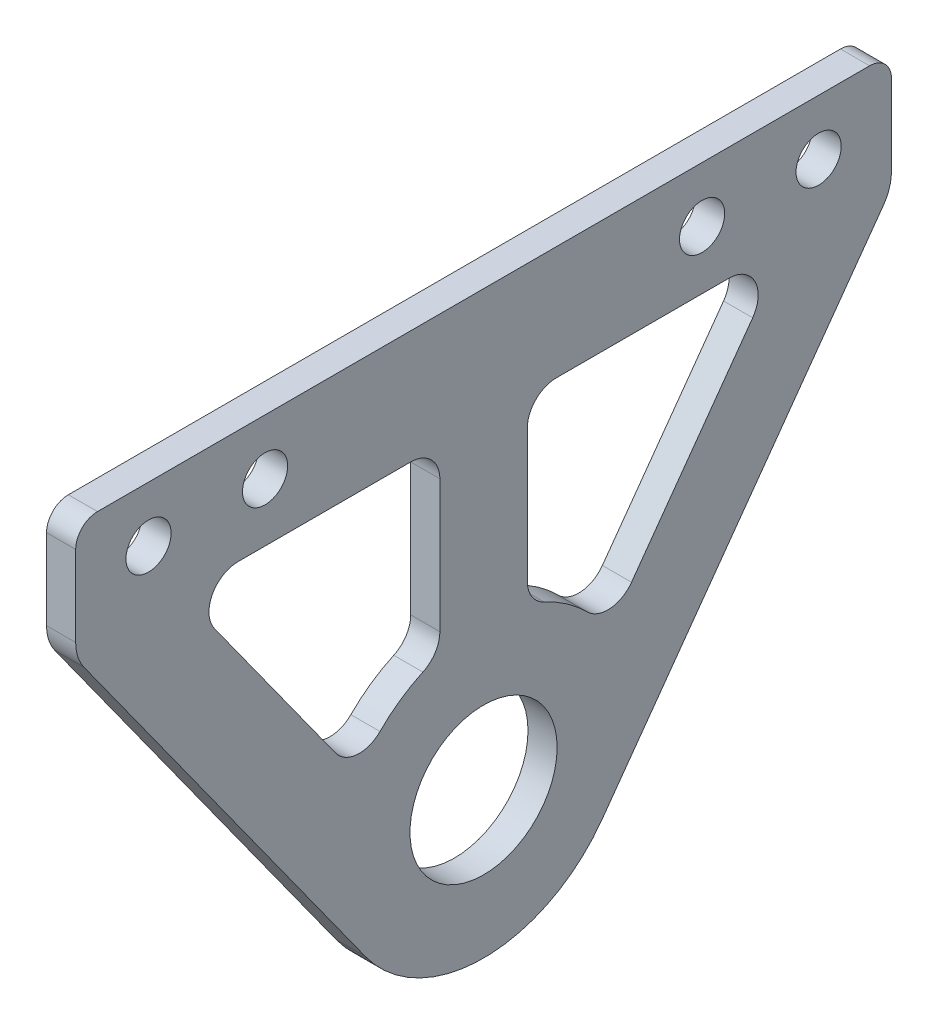
from build123d import *

# Parameters (mm, degrees)
SKETCH_1_R          = 5.05
SKETCH_1_R_2        = 1.55
EXTRUDE_1_DEPTH     = 2
CUT_EXTRUDE_1_DEPTH = 41.93946751
FILLET_1_R          = 2
FILLET_2_R          = 2
FILLET_3_R          = 3
FILLET_4_R          = 1.5


with BuildPart() as part:
    # 草图1 → 凸台-拉伸1 (new body)
    with BuildSketch(Plane(origin=(0, 0, 0), x_dir=(0, 0, -1), z_dir=(1, 0, 0))):
        with BuildLine():
            Line((-28, 29.8), (-28, 21.8))
            Line((-28, 21.8), (-8.117896343, -5.83949989))
            ThreePointArc((-8.117896343, -5.83949989), (0, -10), (8.117896343, -5.83949989))
            Line((8.117896343, -5.83949989), (28, 21.8))
            Line((28, 21.8), (28, 29.8))
            Line((28, 29.8), (-28, 29.8))
        make_face()
        Circle(SKETCH_1_R, mode=Mode.SUBTRACT)
        with Locations((-15, 26)):
            Circle(SKETCH_1_R_2, mode=Mode.SUBTRACT)
        with Locations((-23, 26)):
            Circle(SKETCH_1_R_2, mode=Mode.SUBTRACT)
        with Locations(Location((23, 26, 0), (0, 0, 180))):
            Circle(SKETCH_1_R_2, mode=Mode.SUBTRACT)
        with Locations(Location((15, 26, 0), (0, 0, 180))):
            Circle(SKETCH_1_R_2, mode=Mode.SUBTRACT)
    extrude(amount=EXTRUDE_1_DEPTH)

    # 草图2 → 切除-拉伸1 (cut, through all)
    with BuildSketch(Plane(origin=(0, 0, 0), x_dir=(0, 0, -1), z_dir=(1, 0, 0))):
        with BuildLine():
            Line((-3, 22), (-3, 9.539392014))
            ThreePointArc((-3, 9.539392014), (-6.209058392, 7.838851566), (-8.599148591, 5.104374939))
            Line((-8.599148591, 5.104374939), (-20.752789943, 22))
            Line((-20.752789943, 22), (-3, 22))
        make_face()
    cut_extrude_1 = extrude(amount=CUT_EXTRUDE_1_DEPTH, mode=Mode.SUBTRACT)

    # 圆角1
    fillet_1_edges = [part.edges().sort_by_distance(p)[0] for p in [
        (1, 22, 3),
        (1, 22, 20.752789943),
        (1, 5.104374939, 8.599148591),
        (1, 9.539392014, 3),
    ]]
    fillet(fillet_1_edges, radius=FILLET_1_R)

    # 镜向1: 切除-拉伸1 across plane
    add(cut_extrude_1.mirror(Plane.XY), mode=Mode.SUBTRACT)

    # 圆角2
    fillet_2_edges = [part.edges().sort_by_distance(p)[0] for p in [
        (1, 22, -20.752789943),
        (1, 22, -3),
        (1, 9.539392014, -3),
        (1, 5.104374939, -8.599148591),
    ]]
    fillet(fillet_2_edges, radius=FILLET_2_R)

    # 圆角3
    fillet_3_edges = [part.edges().sort_by_distance(p)[0] for p in [
        (1, 21.8, -28),
        (1, 21.8, 28),
    ]]
    fillet(fillet_3_edges, radius=FILLET_3_R)

    # 圆角4
    fillet_4_edges = [part.edges().sort_by_distance(p)[0] for p in [
        (1, 29.8, -28),
        (1, 29.8, 28),
    ]]
    fillet(fillet_4_edges, radius=FILLET_4_R)


solid = part.part
